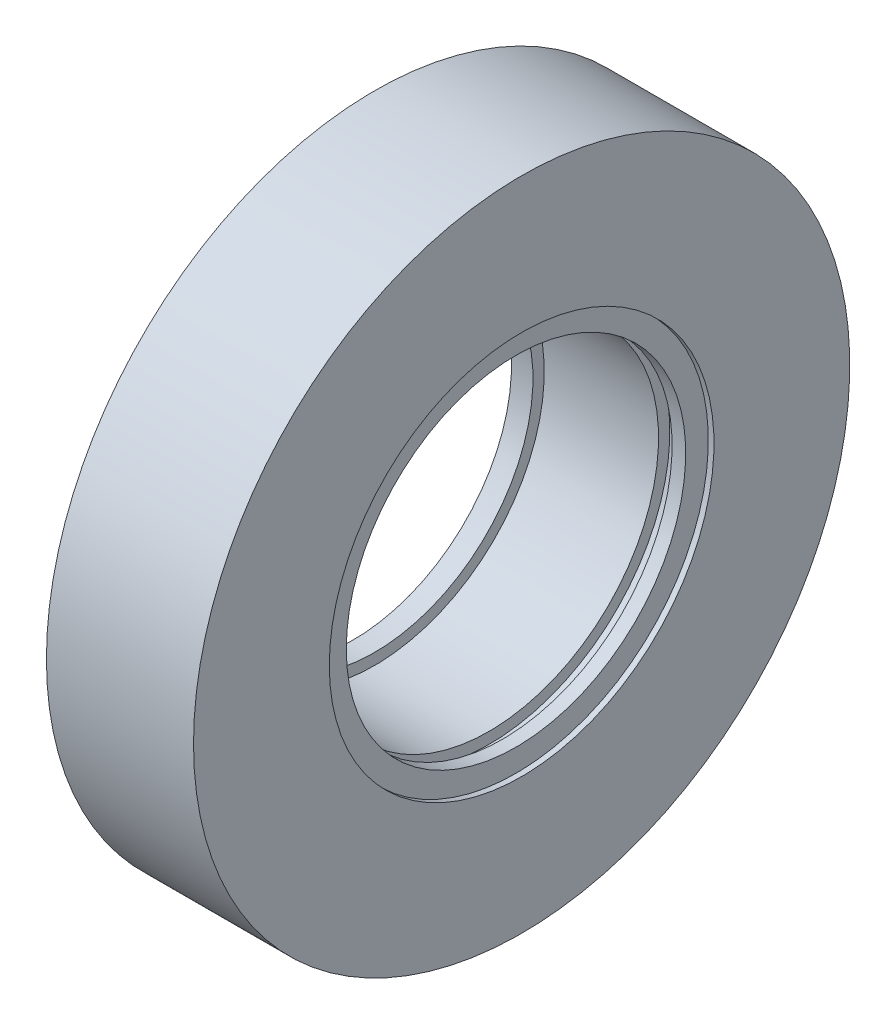
SolidWorks part; units mm, degrees
ref_plane "前视基准面" through (0, 0, 0) normal (0, 0, 1) x (1, 0, 0)
ref_plane "上视基准面" through (0, 0, 0) normal (0, 1, 0) x (1, 0, 0)
ref_plane "右视基准面" through (0, 0, 0) normal (1, 0, 0) x (0, 0, -1)
sketch "草图2" plane through (0, 0, 0) normal (0, 0, 1) x (1, 0, 0)
  line L0 (-10.4961, 0) -> (112.4039, 0) construction
  line L1 (0, 14) -> (1.9, 14)
  line L2 (1.9, 14) -> (1.9, 15)
  line L3 (1.9, 15) -> (12, 15)
  line L4 (12, 15) -> (12, 16)
  line L5 (12, 16) -> (13.2, 16)
  line L6 (13.2, 16) -> (13.2, 15)
  line L7 (13.2, 15) -> (14.4, 15)
  line L8 (14.4, 15) -> (14.4, 17)
  line L9 (14.4, 17) -> (14.9, 17)
  line L10 (14.9, 17) -> (14.9, 29)
  line L11 (14.9, 29) -> (1.9, 29)
  line L12 (1.9, 29) -> (1.9, 25)
  line L13 (1.9, 25) -> (0, 25)
  line L14 (0, 25) -> (0, 14)
  dimension "D1" = 14
  dimension "D2" = 1.9
  dimension "D3" = 1
  dimension "D4" = 10.1
  dimension "D5" = 1
  dimension "D6" = 1.2
  dimension "D7" = 1
  dimension "D8" = 1.2
  dimension "D9" = 2
  dimension "D10" = 0.5
  dimension "D11" = 12
  dimension "D12" = 13
  dimension "D13" = 4
revolve "旋转1" add sketch "草图2" angle 360 about L0
